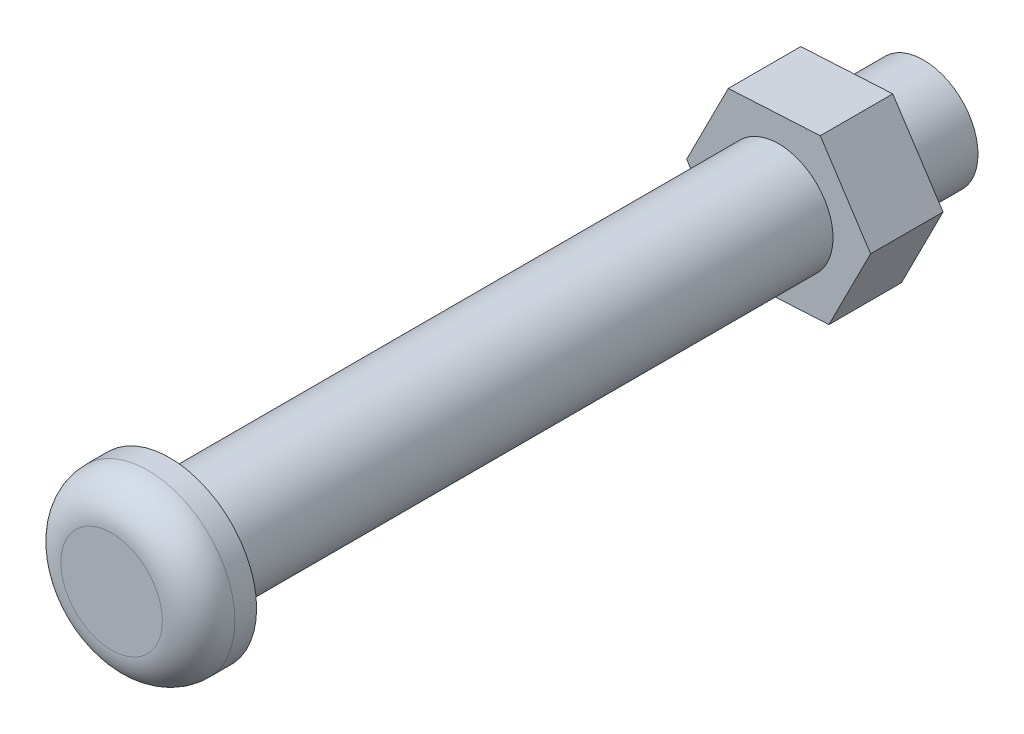
from build123d import *

# Parameters (mm, degrees)
SKETCH1_R           = 4.7625
BOSS_EXTRUDE1_DEPTH = 66.04
SKETCH2_R           = 7.62
BOSS_EXTRUDE2_DEPTH = 5.08
FILLET1_R           = 3.175
SKETCH3_R           = 4.7625
BOSS_EXTRUDE3_DEPTH = 6.35


with BuildPart() as part:
    # Sketch1 → Boss-Extrude1 (new body)
    with BuildSketch(Plane.XY):
        with Locations((-34.925, -76.2)):
            Circle(SKETCH1_R)
    extrude(amount=-BOSS_EXTRUDE1_DEPTH)

    # Sketch2 → Boss-Extrude2 (add)
    with BuildSketch(Plane.XY):
        with Locations((-34.925, -76.2)):
            Circle(SKETCH2_R)
    extrude(amount=BOSS_EXTRUDE2_DEPTH)

    # Fillet1
    fillet1_edges = [part.edges().sort_by_distance(p)[0] for p in [
        (-42.545, -76.2, 5.08),
    ]]
    fillet(fillet1_edges, radius=FILLET1_R)


with BuildPart() as body_2:
    # Sketch3 → Boss-Extrude3 (new body)
    with BuildSketch(Plane(origin=(0, 0, -53.34), x_dir=(-1, 0, 0), z_dir=(0, 0, -1))):
        Polygon((39.331234536, -69.444355652), (31.277557644, -69.006266783), (26.871323108, -75.761911131), (30.518765464, -82.955644348), (38.572442356, -83.393733217), (42.978676892, -76.638088869), align=None)
        with Locations((34.925, -76.2)):
            Circle(SKETCH3_R, mode=Mode.SUBTRACT)
    extrude(amount=BOSS_EXTRUDE3_DEPTH)


solid = Compound([part.part, body_2.part])
